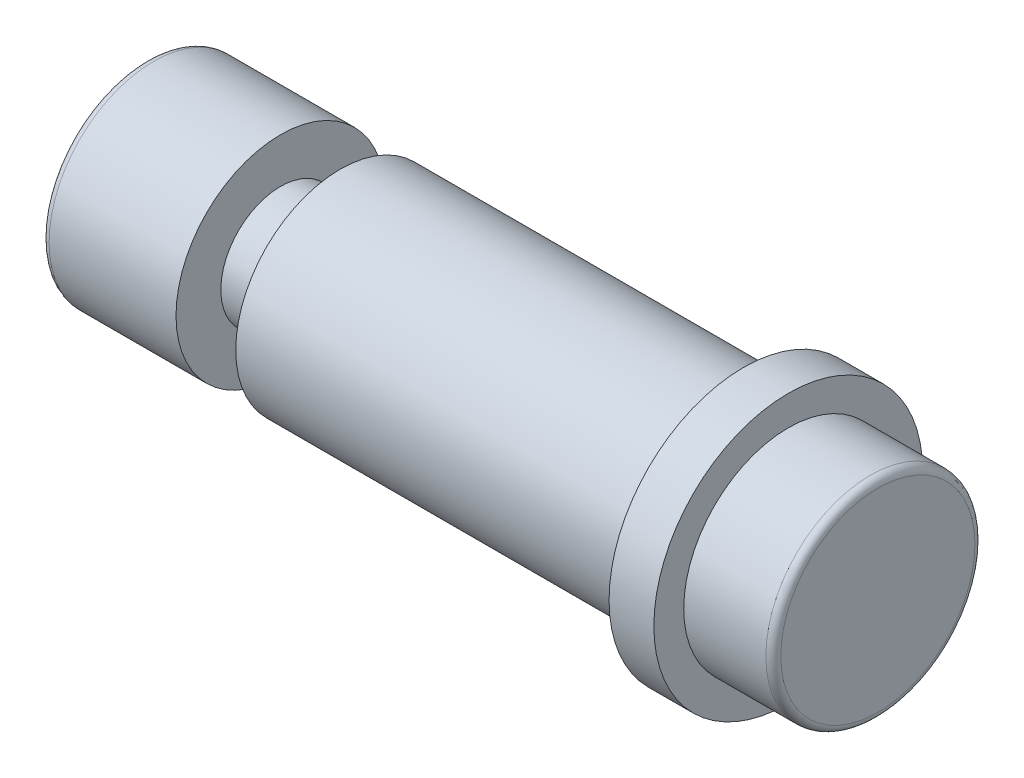
from build123d import *

# Parameters (mm, degrees)
FILLET1_R = 0.5


with BuildPart() as part:
    # Sketch1 → Revolve1 (revolve)
    with BuildSketch(Plane.XY, mode=Mode.PRIVATE) as revolve1_sk:
        Polygon((0, 0), (0, 7), (9, 7), (9, 4), (13, 4), (13, 7), (40, 7), (40, 9), (43, 9), (43, 7), (49, 7), (49, 0), align=None)
    revolve(revolve1_sk.sketch.rotate(Axis((49, 0, 0), (-1, 0, 0)), 90), axis=Axis((49, 0, 0), (-1, 0, 0)))

    # Fillet1
    fillet1_edges = [part.edges().sort_by_distance(p)[0] for p in [
        (0, 0, 7),
        (49, 0, 7),
    ]]
    fillet(fillet1_edges, radius=FILLET1_R)


solid = part.part
